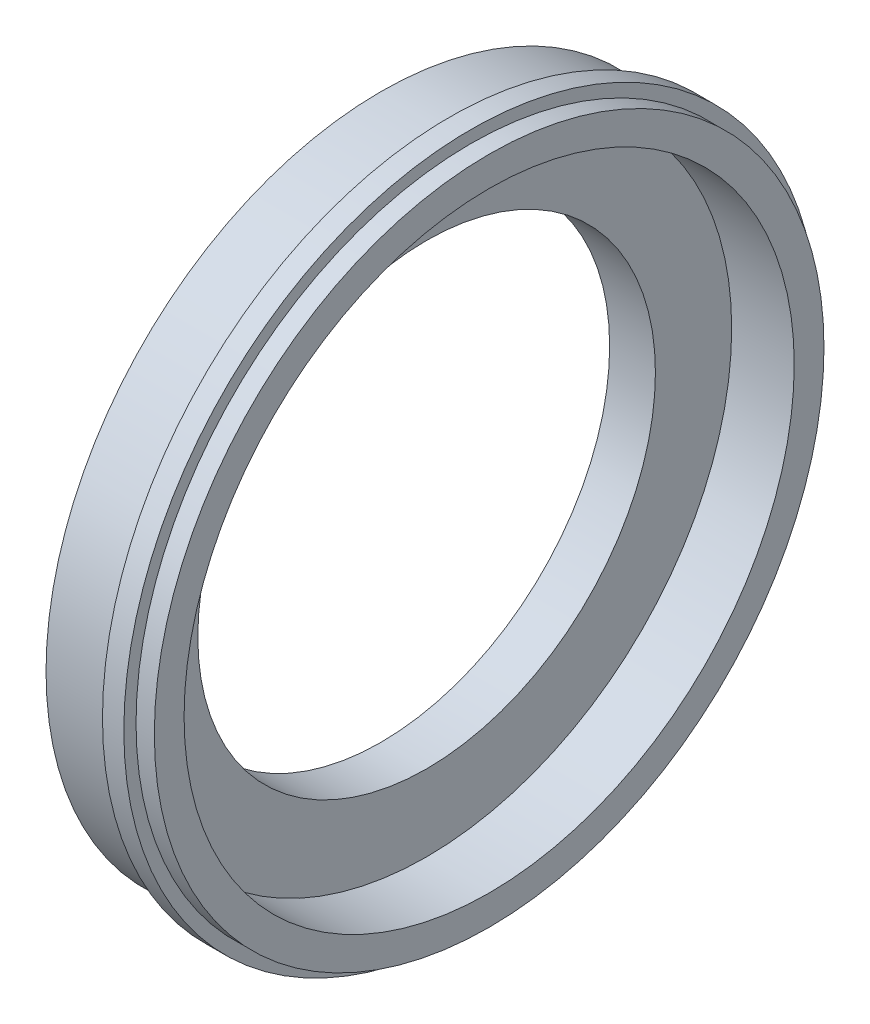
from build123d import *


with BuildPart() as part:
    # Sketch1 → Revolve1 (revolve)
    with BuildSketch(Plane(origin=(0, 0, 0), x_dir=(1, 0, 0), z_dir=(0, 1, 0)), mode=Mode.PRIVATE) as revolve1_sk:
        Polygon((0, 150), (0, 163), (14, 163), (14, 177), (0, 177), (0, 189), (14, 189), (14, 203), (0, 203), (0, 219.5), (45, 219.5), (45, 227.5), (59, 227.5), (59, 219.5), (71, 219.5), (71, 200), (30, 200), (30, 150), align=None)
    revolve(revolve1_sk.sketch.rotate(Axis((0, 0, 0), (1, 0, 0)), 180), axis=Axis((0, 0, 0), (1, 0, 0)))


solid = part.part
